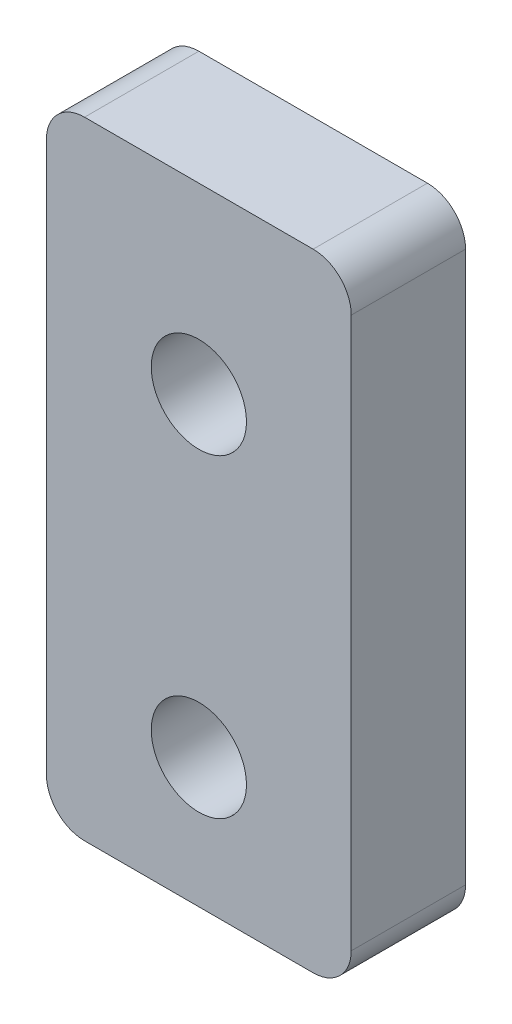
from build123d import *

# Parameters (mm, degrees)
SKETCH_1_W      = 8
SKETCH_1_H      = 16.45
SKETCH_1_R      = 1.25
EXTRUDE_1_DEPTH = 3
FILLET_1_R      = 1


with BuildPart() as part:
    # 草图1 → 凸台-拉伸1 (new body)
    with BuildSketch(Plane.XY):
        with Locations((0, 4.825)):
            Rectangle(SKETCH_1_W, SKETCH_1_H)
        Circle(SKETCH_1_R, mode=Mode.SUBTRACT)
        with Locations((0, 8.25)):
            Circle(SKETCH_1_R, mode=Mode.SUBTRACT)
    extrude(amount=EXTRUDE_1_DEPTH)

    # 圆角1
    fillet_1_edges = [part.edges().sort_by_distance(p)[0] for p in [
        (4, -3.4, 1.5),
        (-4, -3.4, 1.5),
        (-4, 13.05, 1.5),
        (4, 13.05, 1.5),
    ]]
    fillet(fillet_1_edges, radius=FILLET_1_R)


solid = part.part
